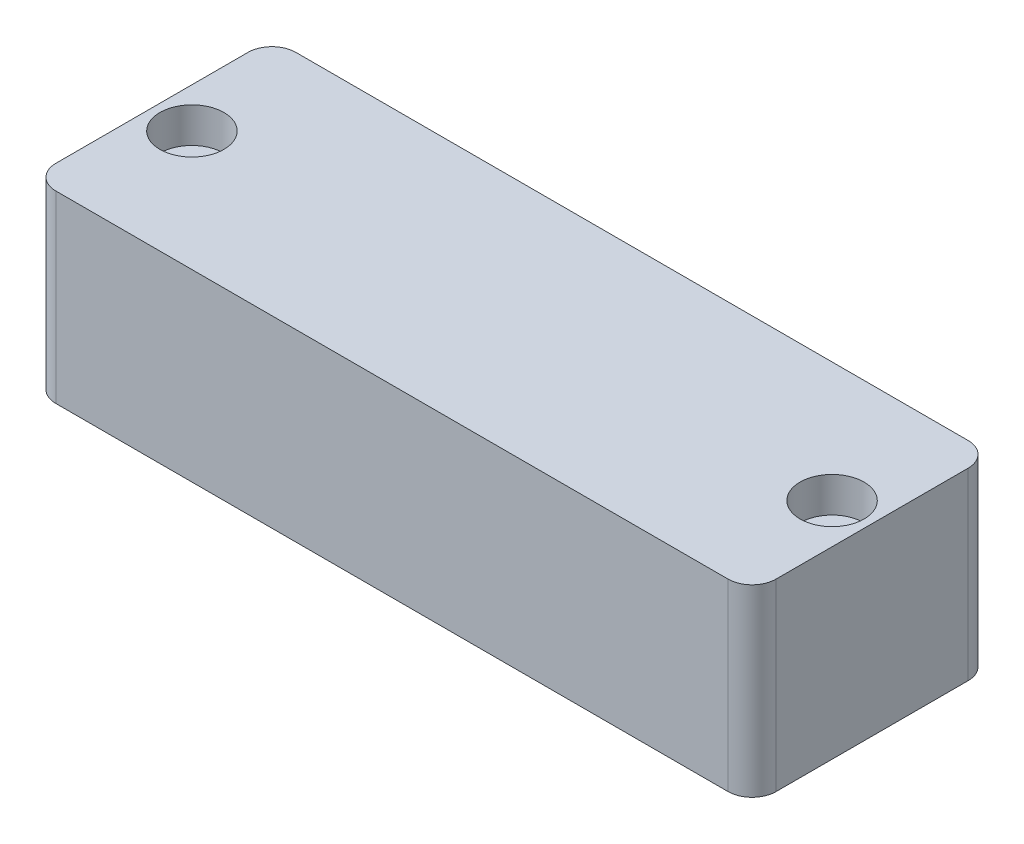
from build123d import *

# Parameters (mm, degrees)
SKETCH_1_W                   = 90
SKETCH_1_H                   = 30
EXTRUDE_1_DEPTH              = 11.5
HOLE_WIZARD_M4_1_D           = 4.5
HOLE_WIZARD_M4_1_CBORE_D     = 8
HOLE_WIZARD_M4_1_CBORE_DEPTH = 4.4
FILLET_1_R                   = 3


with BuildPart() as part:
    # 草图1 → 凸台-拉伸1 (new, symmetric)
    with BuildSketch(Plane(origin=(0, 0, 0), x_dir=(1, 0, 0), z_dir=(0, 1, 0))):
        Rectangle(SKETCH_1_W, SKETCH_1_H)
    extrude(amount=EXTRUDE_1_DEPTH, both=True)

    # M4 六角凹头螺钉的柱形沉头孔1 (through all)
    with Locations(Plane(origin=(0, 11.5, 0), x_dir=(1, 0, 0), z_dir=(0, 1, 0))):
        with Locations((-40, 0), (40, 0)):
            CounterBoreHole(HOLE_WIZARD_M4_1_D / 2, HOLE_WIZARD_M4_1_CBORE_D / 2, HOLE_WIZARD_M4_1_CBORE_DEPTH)

    # 圆角1
    fillet_1_edges = [part.edges().sort_by_distance(p)[0] for p in [
        (45, 0, 15),
        (-45, 0, 15),
        (-45, 0, -15),
        (45, 0, -15),
    ]]
    fillet(fillet_1_edges, radius=FILLET_1_R)


solid = part.part
